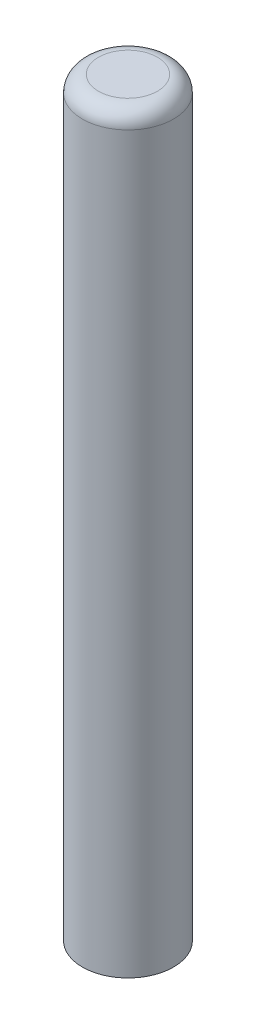
from build123d import *

# Parameters (mm, degrees)
SKETCH1_R           = 4.25
BOSS_EXTRUDE1_DEPTH = 70
FILLET1_R           = 1.5


with BuildPart() as part:
    # Sketch1 → Boss-Extrude1 (new body)
    with BuildSketch(Plane(origin=(0, 0, 0), x_dir=(1, 0, 0), z_dir=(0, 1, 0))):
        with Locations(Location((0, 0, 0), (0, 0, 270))):
            Circle(SKETCH1_R)
    extrude(amount=BOSS_EXTRUDE1_DEPTH)

    # Fillet1
    fillet1_edges = [part.edges().sort_by_distance(p)[0] for p in [
        (0, 70, -4.25),
    ]]
    fillet(fillet1_edges, radius=FILLET1_R)


solid = part.part
